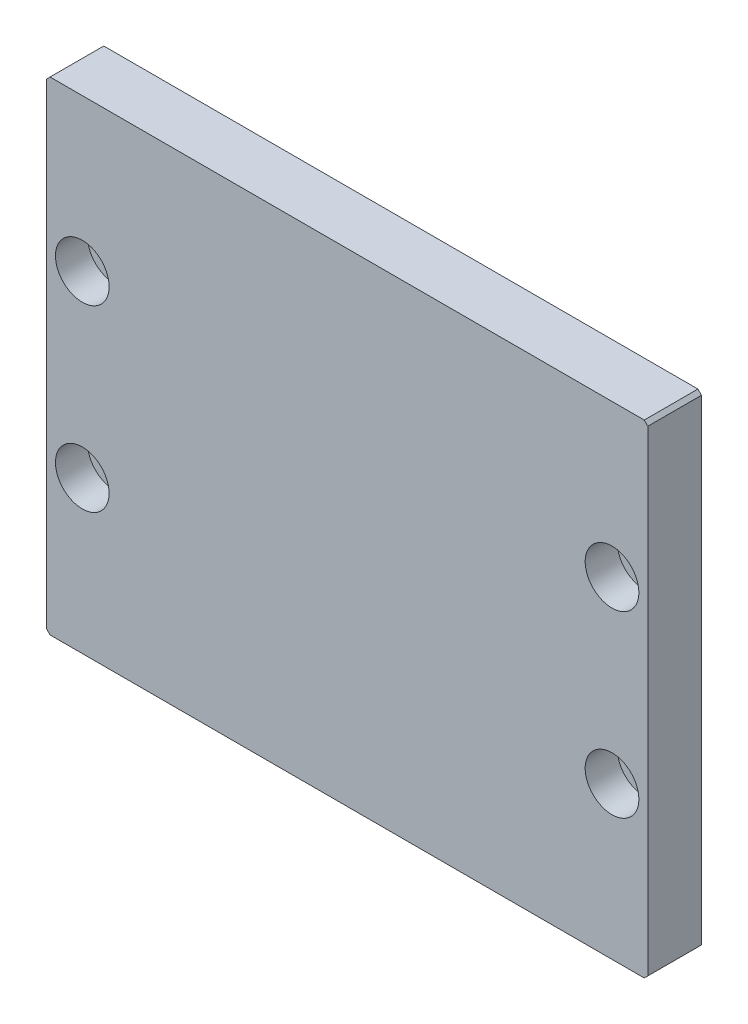
SolidWorks part; units mm, degrees
ref_plane "Front Plane" through (0, 0, 0) normal (0, 0, 1) x (1, 0, 0)
ref_plane "Top Plane" through (0, 0, 0) normal (0, 1, 0) x (1, 0, 0)
ref_plane "Right Plane" through (0, 0, 0) normal (1, 0, 0) x (0, 0, -1)
sketch "Sketch1" plane through (0, 0, 0) normal (0, 0, 1) x (1, 0, 0)
  line L1 (-84, 67.5) -> (84, 67.5)
  line L2 (-84, 67.5) -> (-84, -67.5)
  line L3 (-84, -67.5) -> (84, -67.5)
  line L4 (84, 67.5) -> (84, -67.5)
  line L5 (-84, 67.5) -> (84, -67.5) construction
  line L6 (-84, -67.5) -> (84, 67.5) construction
  point P0 (0, 0)
  dimension "D1" = 168
  dimension "D2" = 135
extrude "Boss-Extrude1" add sketch "Sketch1" along normal blind 15
hole_wizard "Hole size per socket head cap screw type1" positions "Sketch3" profile "Sketch2" counterbore size "M8" standard "GB" end condition through all
sketch "Sketch3" plane through (0, 0, 15) normal (0, 0, 1) x (1, 0, 0)
  line L0 (0, 67.5) -> (0, -67.5) construction
  line L1 (84, 67.5) -> (-84, 67.5) construction
  line L2 (-84, -67.5) -> (84, -67.5) construction
  line L4 (-84, 0) -> (84, 0) construction
  line L5 (-84, 67.5) -> (-84, -67.5) construction
  line L6 (84, -67.5) -> (84, 67.5) construction
  point P0 (-74, 25)
  point P1 (-74, -25)
  point P3 (74, -25)
  point P5 (74, 25)
  dimension "D1" = 148
  dimension "D2" = 50
sketch "Sketch2" plane through (-74, 25, 15) normal (1, 0, 0) x (0, -1, 0)
  line L0 (0, 0) -> (0, 15)
  line L1 (0, 15) -> (4.5, 15)
  line L3 (4.5, 15) -> (4.5, 9)
  line L4 (4.5, 9) -> (7.5, 9)
  line L5 (7.5, 9) -> (7.5, 0)
  line L7 (7.5, 0) -> (0, 0)
  line L11 (0, -6.35) -> (0, 107.95) construction
  dimension "通孔孔直径" = 9
  dimension "通孔孔深度" = 15
  dimension "柱形沉头孔直径" = 15
  dimension "柱形沉头孔深度" = 9
chamfer "Chamfer1" distance 1 angle 45 4 edges at (-84, 67.5, 7.5) (84, 67.5, 7.5) (84, -67.5, 7.5) (-84, -67.5, 7.5)
